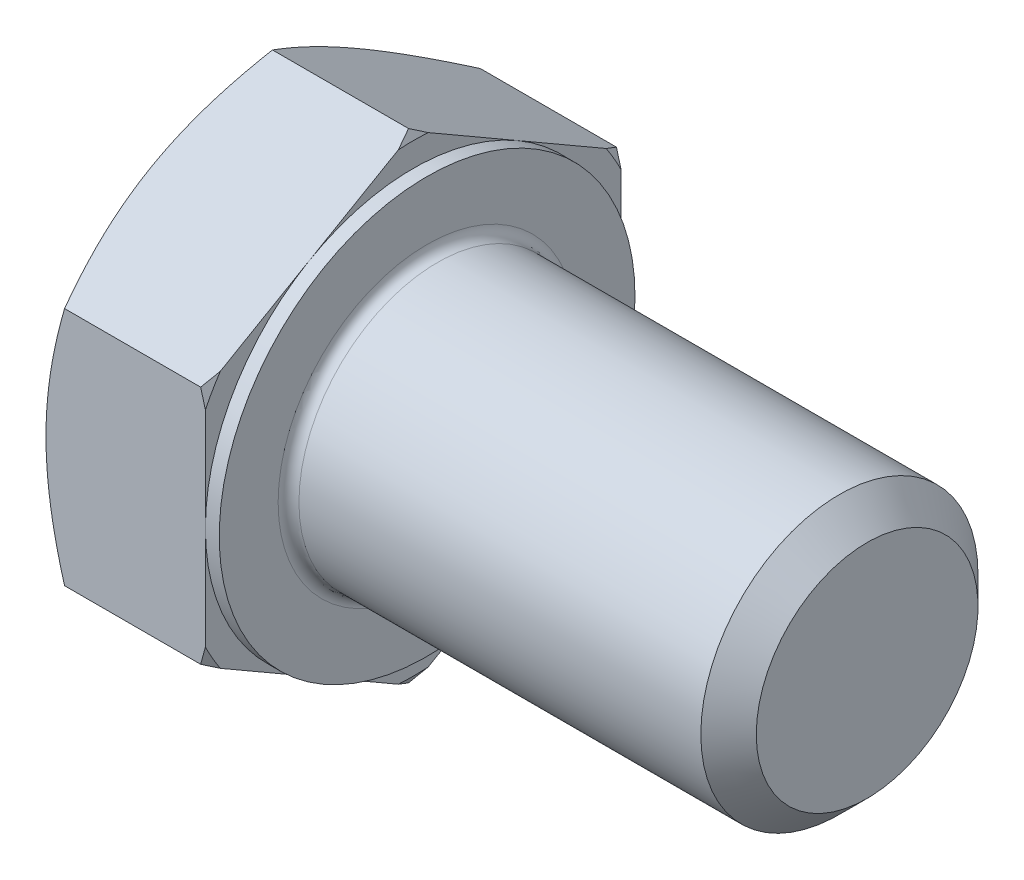
SolidWorks part; units mm, degrees
material "SAE2"
ref_plane "Front" through (0, 0, 0) normal (0, 0, 1) x (1, 0, 0)
ref_plane "Top" through (0, 0, 0) normal (0, 1, 0) x (1, 0, 0)
ref_plane "Right" through (0, 0, 0) normal (1, 0, 0) x (0, 0, -1)
sketch "Sketch1" plane through (0, 0, 0) normal (1, 0, 0) x (0, 0, -1)
  line L0 (12, 6.9282) -> (12, -6.9282)
  line L1 (-12, 6.9282) -> (-12, -6.9282)
  line L2 (12, -6.9282) -> (0, -13.8564)
  line L3 (0, -13.8564) -> (-12, -6.9282)
  line L4 (12, 6.9282) -> (0, 13.8564)
  line L5 (0, 13.8564) -> (-12, 6.9282)
  dimension "s" = 24
  dimension "D2" = 120
  dimension "D3" = 12
  dimension "D4" = 12
  dimension "D5" = 12
extrude "Base-Extrude" add sketch "Sketch1" along normal blind 10
sketch "Sketch2" plane through (0, 0, 0) normal (0, 0, 1) x (1, 0, 0)
  line L0 (0, 6.9282) -> (0, -6.9282) construction
  line L1 (0, 0) -> (35.4, 0)
  line L2 (0, 0) -> (0, 8)
  line L3 (0, 8) -> (27.8072, 8)
  line L4 (35.4, 0) -> (35.4, 6.268)
  line L5 (10, 13.8564) -> (10, 6.9282) construction
  line L7 (0, 0) -> (96.52, 0) construction
  line L8 (35.4, -6.268) -> (27.8072, -8) construction
  line L9 (0, -8) -> (27.8072, -8) construction
  line L10 (12, 15.24) -> (12, -1.27) construction
  line L11 (10, 15.24) -> (10, -1.27) construction
  line L12 (10, 6.9282) -> (10, -6.9282) construction
  line L13 (27.8072, 8) -> (35.4, 8)
  line L14 (35.4, 8) -> (35.4, 6.268)
  dimension "l" = 25.4
  dimension "m" = 16
  dimension "Minor_dia" = 12.536
  dimension "p" = 2
  dimension "h" = 25.4
revolve "Boss-Revolve1" add sketch "Sketch2" angle 360 about L7
cosmetic thread "Helix1" parameters "Thread_length"=36, "Thread_minor"=12.536
sketch "Sketch3" plane through (0, 0, 0) normal (0, 0, 1) x (1, 0, 0)
  line L0 (0, 12) -> (3.9585, 18.8564)
  line L1 (0, 13.8564) -> (0, 6.9282) construction
  line L2 (3.9585, 18.8564) -> (3.9585, 23.8564)
  line L3 (3.9585, 23.8564) -> (-10, 23.8564)
  line L4 (-10, 23.8564) -> (-10, 12)
  line L5 (-10, 12) -> (0, 12)
  line L6 (0, 0) -> (99.06, 0) construction
  line L7 (10, 13.8564) -> (0, 13.8564) construction
  dimension "D1" = 12
  dimension "D2" = 5
  dimension "D3" = 10
  dimension "D4" = 5
  dimension "Head_ch_ang" = 30
revolve "Cut-Revolve1" cut sketch "Sketch3" angle 360 about L6
sketch "Sketch5" plane through (0, 0, 0) normal (0, 0, 1) x (1, 0, 0)
  line L0 (10, 12) -> (6.0415, 18.8564)
  line L1 (10, 13.8564) -> (10, 6.9282) construction
  line L2 (6.0415, 18.8564) -> (6.0415, 23.8564)
  line L3 (6.0415, 23.8564) -> (16.0415, 23.8564)
  line L4 (16.0415, 23.8564) -> (16.0415, 12)
  line L5 (16.0415, 12) -> (10, 12)
  line L7 (10, 13.8564) -> (1.0718, 13.8564) construction
  line L8 (0, 0) -> (99.06, 0) construction
  line L9 (0, 0) -> (99.06, 0) construction
  dimension "D1" = 12
  dimension "D2" = 5
  dimension "D3" = 10
  dimension "Head_ch_ang" = 30
  dimension "D4" = 5
revolve "Cut-Revolve2" cut sketch "Sketch5" angle 360 about L8
sketch "Sketch4" plane through (0, 0, 0) normal (0, 0, 1) x (1, 0, 0)
  line L1 (10, 13.8564) -> (10, 6.9282) construction
  line L2 (10, 12) -> (9.2, 12)
  line L3 (10, 12) -> (10, 23.8564)
  line L4 (10, 23.8564) -> (9.2, 23.8564)
  line L5 (0, 0) -> (95.25, 0) construction
  line L6 (0, 0) -> (96.52, 0) construction
  line L7 (9.2, 12) -> (9.2, 23.8564)
  line L8 (8.9282, 13.8564) -> (1.0718, 13.8564) construction
  dimension "D1" = 24
  dimension "D2" = 10
  dimension "c" = 0.8
revolve "Cut-Revolve3" cut sketch "Sketch4" angle 360 about L5
chamfer "Chamfer" distance 1.6 angle 45 1 edges at (35.4, 0, 8)
fillet "Fillet" radius 0.6 1 edges at (10, 0, -8)
sketch "Sketch6" plane through (0, 0, 0) normal (0, 0, 1) x (1, 0, 0)
  line L0 (12, -6.268) -> (11, -8)
  line L1 (12, -6.268) -> (13, -8)
  line L2 (13, -8) -> (13, -10)
  line L3 (-3.175, 0) -> (5.1513, 0) construction
  line L5 (13, -10) -> (11, -10)
  line L6 (11, -10) -> (11, -8)
  dimension "Thread_minor" = 12.536
  dimension "Diameter" = 16
  dimension "Start" = 12
  dimension "SideAngle" = 60
  dimension "VeeAngle" = 60
  dimension "Overcut" = 20
revolve "Cut-Revolve4" [suppressed] cut sketch "Sketch6" angle 360 about L3
pattern_linear "LPattern1" [suppressed]
